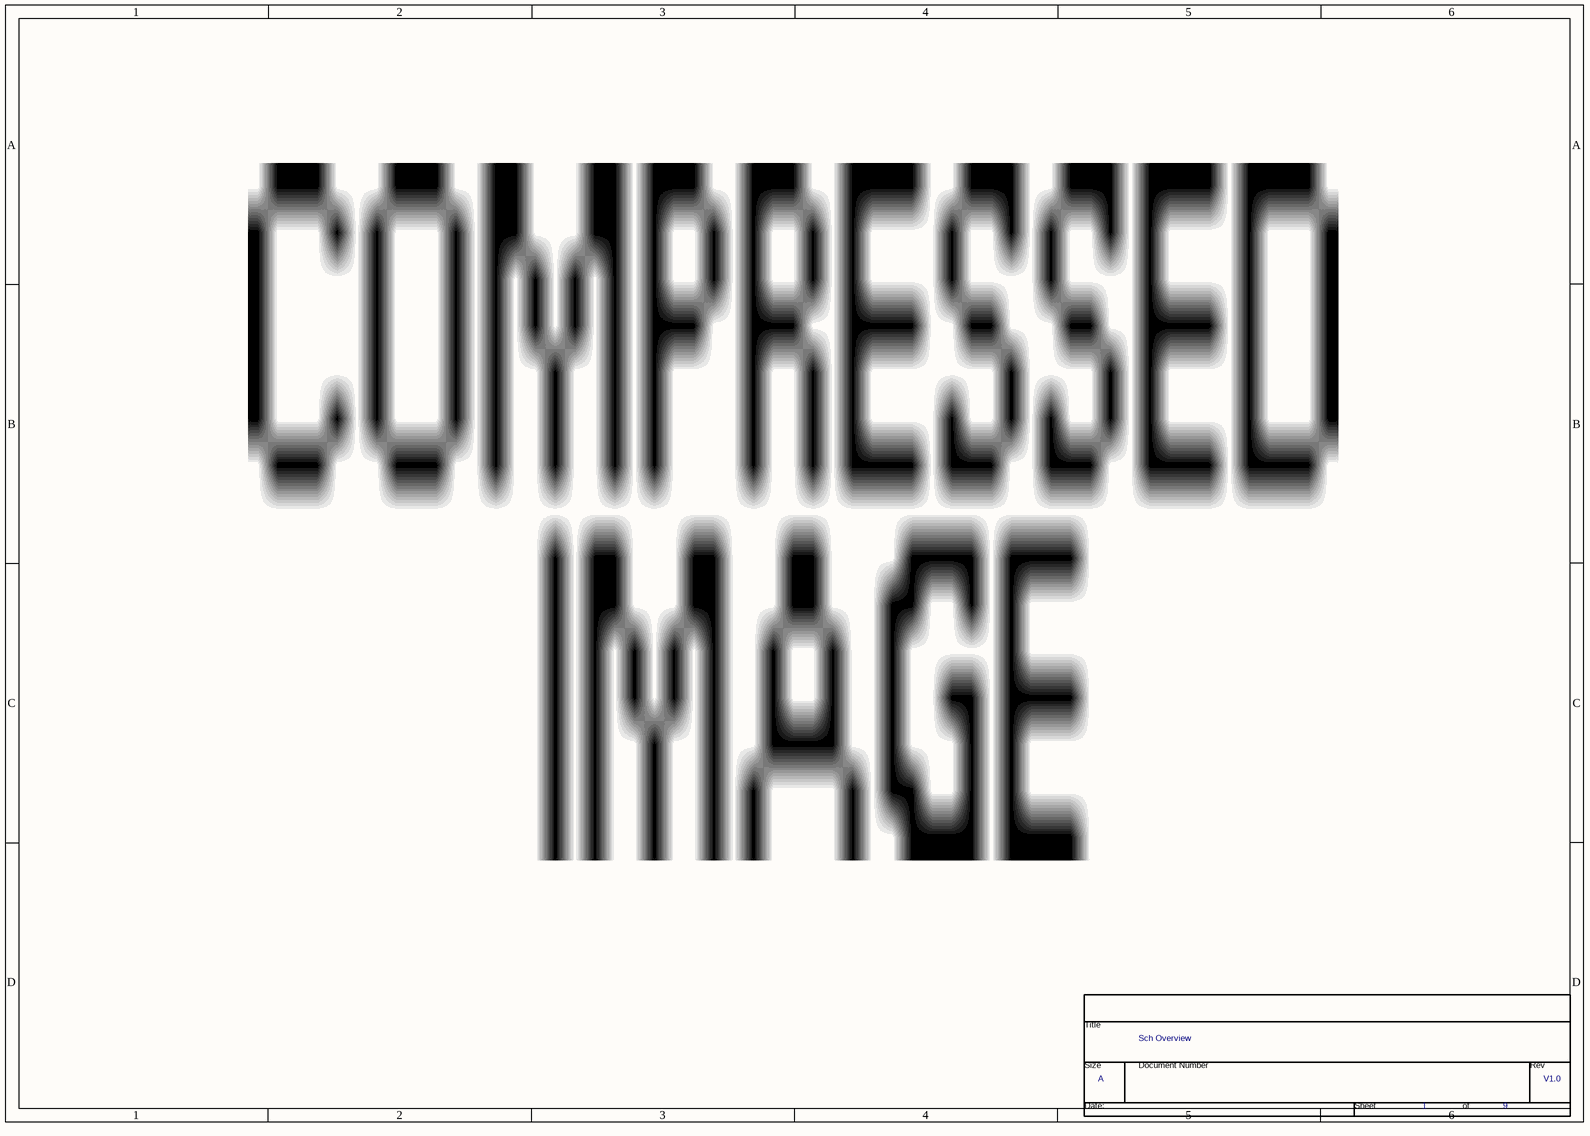
[diagram p0: MISC86294-2.SchDoc]
# Altium project MISC86294-22.PrjPcb (part 1 of 5)
9 sheets, 321 parts. Net scope: flat (ports and power ports of the same name join across sheets).
Board file: MISC86294.PcbDoc
Sheets:
  MISC86294-2.SchDoc
  MISC86294-4.SchDoc
  MISC86294-6.SchDoc
  MISC86294-8.SchDoc
  MISC86294-10.SchDoc
  MISC86294-12.SchDoc
  MISC86294-14.SchDoc
  MISC86294-16.SchDoc
  MISC86294-18.SchDoc

## Sheet MISC86294-2.SchDoc
size 297 x 209 mm

### Parts
(Parts that share a designator on the sheet are numbered #1, #2 ... from top to bottom, then left to right.)
*#1  RevCode: V1.0  Title: Sch Overview  Page Size: A  Page Number: 1  Page Count: 9  (hidden comment: TitleBlock0)  (graphical)

### Library data of the parts
*#1 = TitleBlock0: Document: Agr-Ctrl-3GS-01; Page Create Date: March  8, 1995

## Sheet MISC86294-4.SchDoc
size 297 x 209 mm
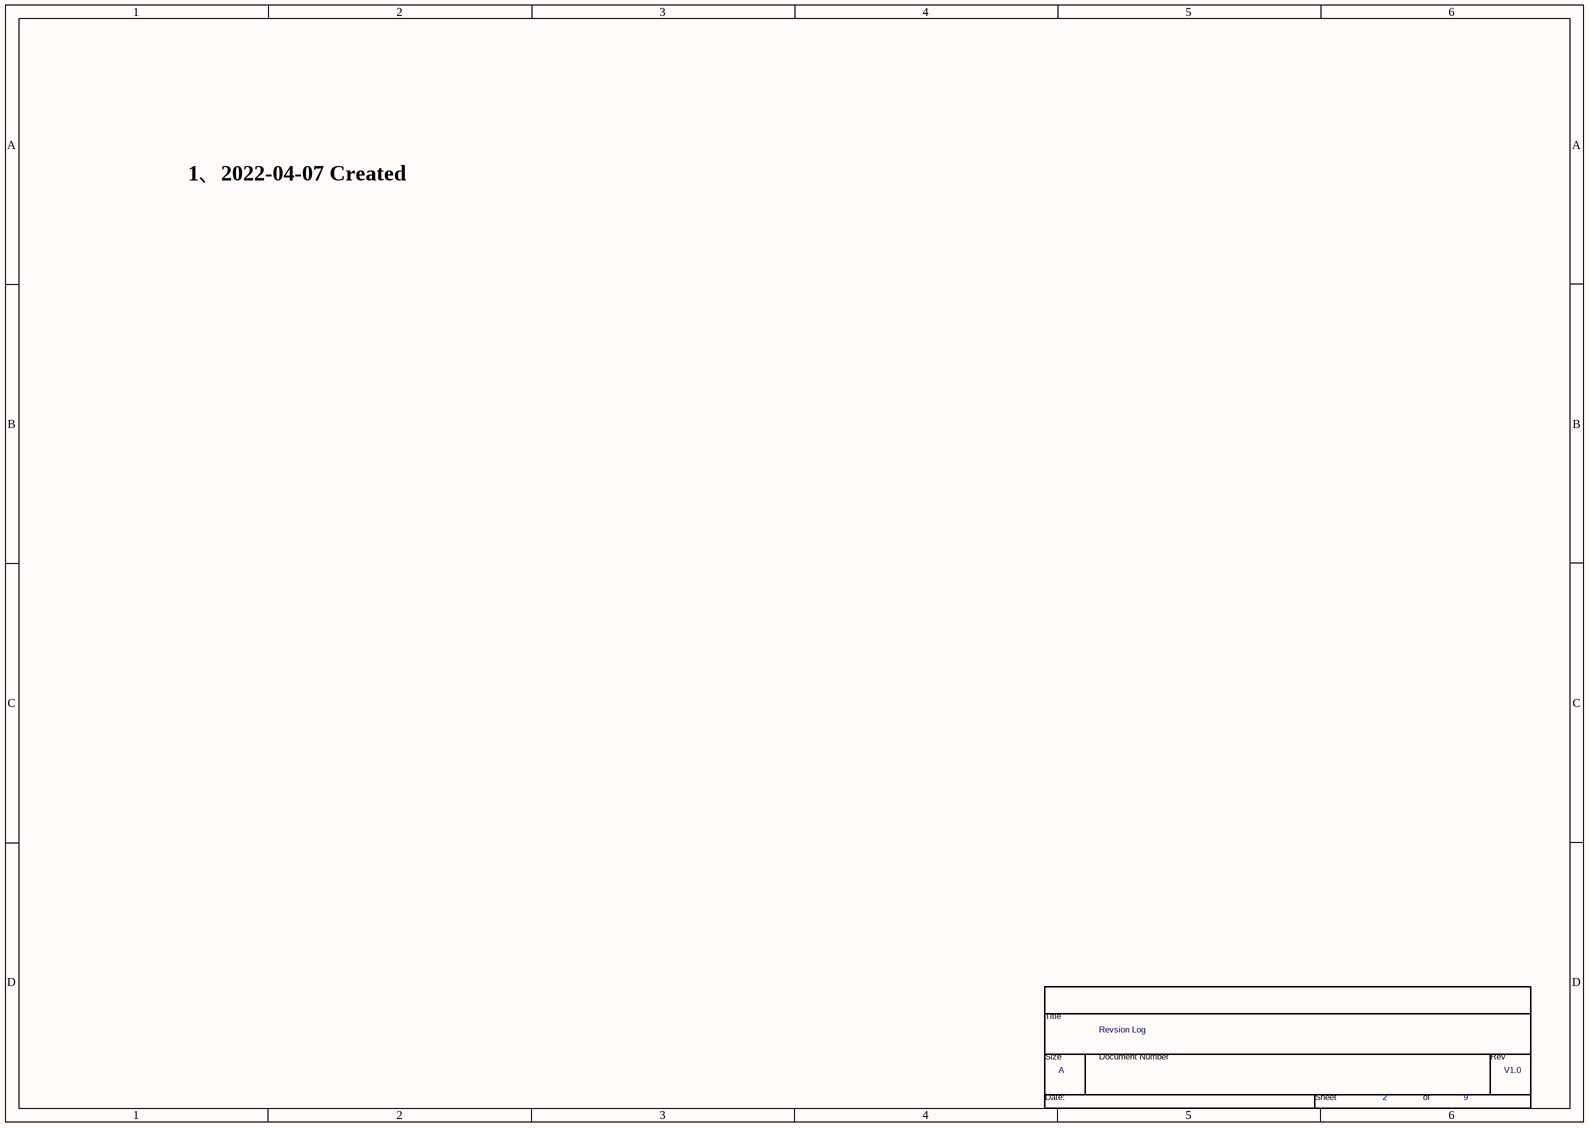
[diagram p1: MISC86294-4.SchDoc]

### Parts
(Parts that share a designator on the sheet are numbered #1, #2 ... from top to bottom, then left to right.)
*#2  RevCode: V1.0  Title: Revsion Log  Page Size: A  Page Number: 2  Page Count: 9  (hidden comment: TitleBlock0)  (graphical)

### Notes on the sheet
- 1、2022-04-07 Created

### Library data of the parts
*#2 = TitleBlock0: Document: Agr-Ctrl-3GS-02; Page Create Date: March  8, 1995

## Sheet MISC86294-6.SchDoc
size 297 x 209 mm
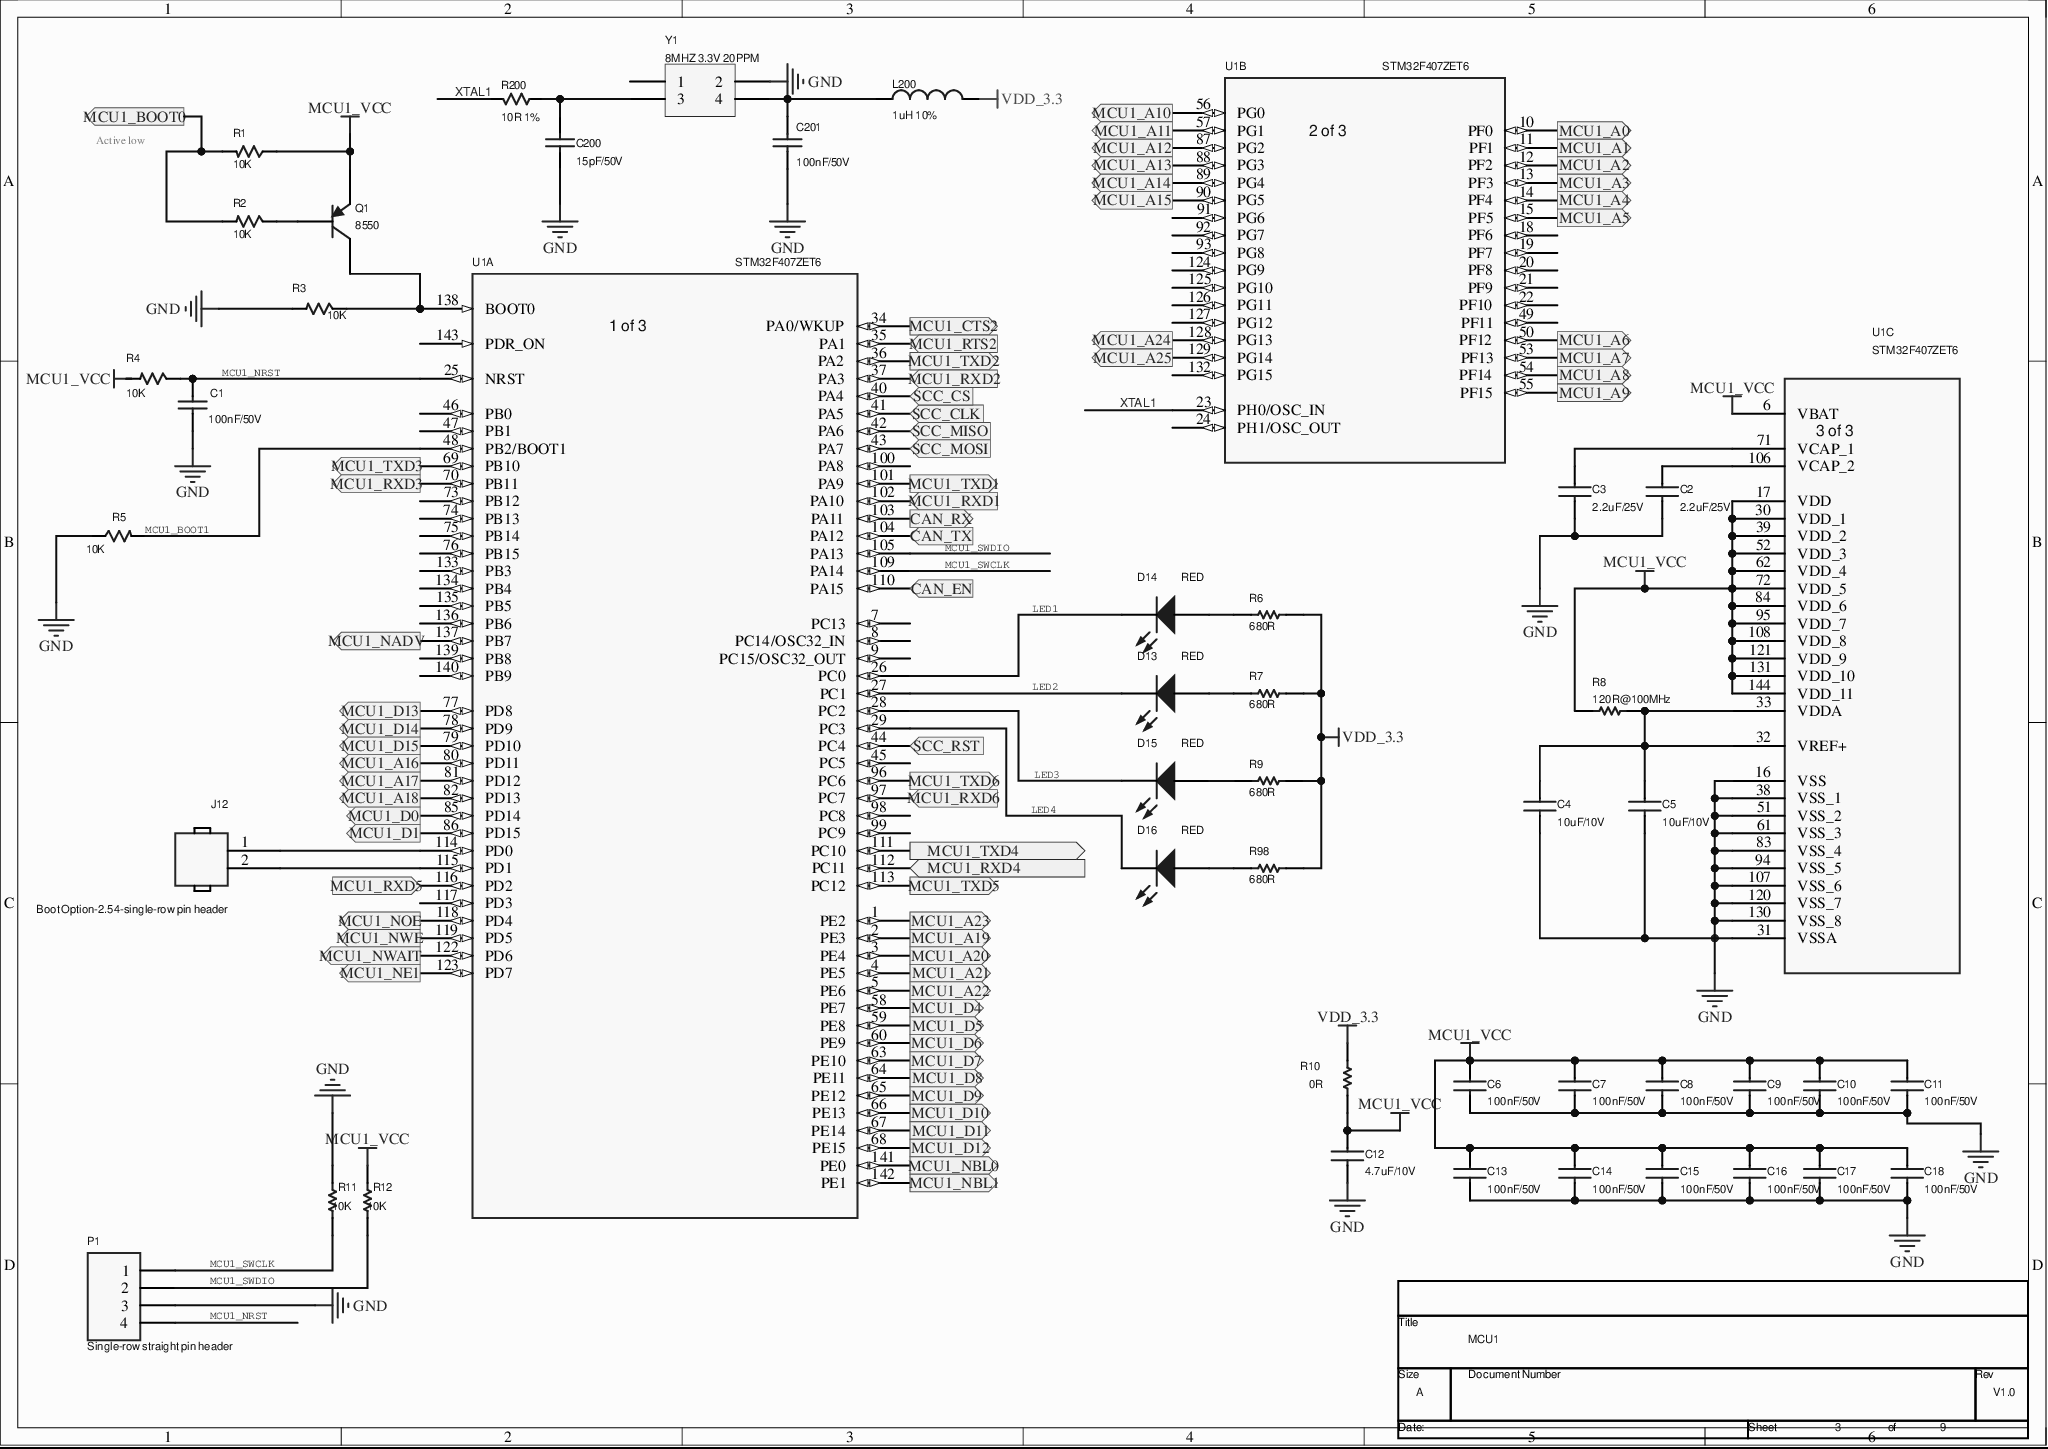
[diagram p2: MISC86294-6.SchDoc]

### Parts
(Parts that share a designator on the sheet are numbered #1, #2 ... from top to bottom, then left to right.)
*#3  RevCode: V1.0  Title: MCU1  Page Size: A  Page Number: 3  Page Count: 9  (hidden comment: TitleBlock0)  (graphical)
C1  100nF/50V  [0603]
C2  2.2uF/25V  [C0603]
C3  2.2uF/25V  [C0603]
C4  10uF/10V  [C0603]
C5  10uF/10V  [C0603]
C6  100nF/50V  [C0603]
C7  100nF/50V  [C0603]
C8  100nF/50V  [C0603]
C9  100nF/50V  [C0603]
C10  100nF/50V  [C0603]
C11  100nF/50V  [C0603]
C12  4.7uF/10V  [C0805]
C13  100nF/50V  [C0603]
C14  100nF/50V  [C0603]
C15  100nF/50V  [C0603]
C16  100nF/50V  [C0603]
C17  100nF/50V  [C0603]
C18  100nF/50V  [C0603]
C200  15pF/50V  [C0603]
C201  100nF/50V  [C0603]
D13  RED  [LED_0805]
D14  RED  [LED_0805]
D15  RED  [LED_0805]
D16  RED  [LED_0805]
J12  Boot Option-2.54-single-row pin header  [HDR_1X2_254]
L200  1uH 10%  [SMD_L6.0-W6.0]
P1  Single-row straight pin header  [HDR1X4]
Q1  8550  [SOT-23-SS8550]
R1  10K  [0603]
R2  10K  [0603]
R3  10K  [0603]
R4  10K  [0603]
R5  10K  [0603]
R6  User_Value: 680R  [0603]  (hidden comment: NA)
R7  User_Value: 680R  [0603]  (hidden comment: NA)
R8  120R@100MHz  [0603]
R9  User_Value: 680R  [0603]  (hidden comment: NA)
R10  0R  [0603]
R11  10K  [0603]
R12  10K  [0603]
R98  User_Value: 680R  [0603]  (hidden comment: NA)
R200  10R 1%  [R0805]
U1  STM32F407ZET6  [LQFP144-20x20mm]  (parts A,B,C of 3)
Y1  8MHZ 3.3V 20PPM  [XTAL 5.7X7.0-SM - duplicate]

### Ports
CAN_EN (in), CAN_RX (out), CAN_TX (in), MCU1_A0 (out), MCU1_A1 (out), MCU1_A2 (out), MCU1_A3 (out), MCU1_A4 (out), MCU1_A5 (out), MCU1_A6 (out), MCU1_A7 (out), MCU1_A8 (out), MCU1_A9 (out), MCU1_A10 (out), MCU1_A11 (out), MCU1_A12 (out), MCU1_A13 (out), MCU1_A14 (out), MCU1_A15 (out), MCU1_A16 (out), MCU1_A17 (out), MCU1_A18 (out), MCU1_A19 (out), MCU1_A20 (out), MCU1_A21 (out), MCU1_A22 (out), MCU1_A23 (out), MCU1_A24 (out), MCU1_A25 (out), MCU1_BOOT0 (out), MCU1_CTS2 (out), MCU1_D0 (out), MCU1_D1 (out), MCU1_D4 (out), MCU1_D5 (out), MCU1_D6 (out), MCU1_D7 (out), MCU1_D8 (out), MCU1_D9 (out), MCU1_D10 (out), MCU1_D11 (out), MCU1_D12 (out), MCU1_D13 (out), MCU1_D14 (out), MCU1_D15 (out), MCU1_NADV (out), MCU1_NBL0 (out), MCU1_NBL1 (out), MCU1_NE1 (out), MCU1_NOE (out), MCU1_NWAIT (out), MCU1_NWE (out), MCU1_RTS2 (in), MCU1_RXD1 (in), MCU1_RXD2 (in), MCU1_RXD3 (out), MCU1_RXD4 (in), MCU1_RXD5 (in), MCU1_RXD6 (in), MCU1_TXD1 (out), MCU1_TXD2 (out), MCU1_TXD3 (out), MCU1_TXD4 (out), MCU1_TXD5 (out), MCU1_TXD6 (out), SCC_CLK (in), SCC_CS (in), SCC_MISO (in), SCC_MOSI (in), SCC_RST (in)

### Nets
GND: C1.1 C2.2 C3.2 C4.2 C5.2 C6.2 C7.2 C8.2 C9.2 C10.2 C11.2 C12.2 C13.2 C14.2 C15.2 C16.2 C17.2 C18.2 C200.1 C201.2 P1.3 R3.1 R5.1 R11.2 U1.16(VSS) U1.31(VSSA) U1.38(VSS_1) U1.51(VSS_2) U1.61(VSS_3) U1.83(VSS_4) U1.94(VSS_5) U1.107(VSS_6) U1.120(VSS_7) U1.130(VSS_8) Y1.2
MCU1_VCC: C6.1 C7.1 C8.1 C9.1 C10.1 C11.1 C12.1 C13.1 C14.1 C15.1 C16.1 C17.1 C18.1 Q1.2(E) R1.2 R4.2 R8.1 R10.2 R12.2 U1.6(VBAT) U1.17(VDD) U1.30(VDD_1) U1.39(VDD_2) U1.52(VDD_3) U1.62(VDD_4) U1.72(VDD_5) U1.84(VDD_6) U1.95(VDD_7) U1.108(VDD_8) U1.121(VDD_9) U1.131(VDD_10) U1.144(VDD_11)
VDD_3.3: L200.2 R6.1 R7.1 R9.1 R10.1 R98.1
IMU_RXD1: U1.111(PC10) ; port MCU1_TXD4
IMU_TXD1: U1.112(PC11) ; port MCU1_RXD4
LED1: D14.2(K) U1.26(PC0)
LED2: D13.2(K) U1.27(PC1)
LED3: D15.2(K) U1.28(PC2)
LED4: D16.2(K) U1.29(PC3)
MCU1_BOOT1: R5.2 U1.48(PB2/BOOT1)
MCU1_NRST: C1.2 P1.4 R4.1 U1.25(NRST)
MCU1_SWCLK: P1.1 R11.1 U1.109(PA14)
MCU1_SWDIO: P1.2 R12.1 U1.105(PA13)
XTAL1: R200.1 U1.23(PH0/OSC_IN)
NetC2_1: C2.1 U1.106(VCAP_2)
NetC3_1: C3.1 U1.71(VCAP_1)
NetC4_1: C4.1 C5.1 R8.2 U1.32(VREF+) U1.33(VDDA)
NetC200_2: C200.2 R200.2 Y1.3
NetC201_1: C201.1 L200.1 Y1.4
NetD13_1: D13.1(A) R7.2
NetD14_1: D14.1(A) R6.2
NetD15_1: D15.1(A) R9.2
NetD16_1: D16.1(A) R98.2
NetJ6_39: U1.116(PD2) ; port MCU1_RXD5
NetJ6_40: U1.113(PC12) ; port MCU1_TXD5
NetJ12_1: J12.1 U1.114(PD0)
NetJ12_2: J12.2 U1.115(PD1)
NetJ13_1: U1.101(PA9) ; port MCU1_TXD1
NetJ13_2: U1.102(PA10) ; port MCU1_RXD1
NetJ14_1: U1.36(PA2) ; port MCU1_TXD2
NetJ14_2: U1.37(PA3) ; port MCU1_RXD2
NetJ16_1: U1.69(PB10) ; port MCU1_TXD3
NetJ16_2: U1.70(PB11) ; port MCU1_RXD3
NetJ22_1: U1.96(PC6) ; port MCU1_TXD6
NetJ22_2: U1.97(PC7) ; port MCU1_RXD6
NetP3_11: R1.1 R2.2 ; port MCU1_BOOT0
NetQ1_1: Q1.1(B) R2.1
NetQ1_3: Q1.3(C) R3.2 U1.138(BOOT0)
NetR23_1: U1.43(PA7) ; port SCC_MOSI
NetR24_1: U1.42(PA6) ; port SCC_MISO
NetU1_1: U1.1(PE2) ; port MCU1_A23
NetU1_2: U1.2(PE3) ; port MCU1_A19
NetU1_3: U1.3(PE4) ; port MCU1_A20
NetU1_4: U1.4(PE5) ; port MCU1_A21
NetU1_5: U1.5(PE6) ; port MCU1_A22
NetU1_10: U1.10(PF0) ; port MCU1_A0
NetU1_11: U1.11(PF1) ; port MCU1_A1
NetU1_12: U1.12(PF2) ; port MCU1_A2
NetU1_13: U1.13(PF3) ; port MCU1_A3
NetU1_14: U1.14(PF4) ; port MCU1_A4
NetU1_15: U1.15(PF5) ; port MCU1_A5
NetU1_34: U1.34(PA0/WKUP) ; port MCU1_CTS2
NetU1_35: U1.35(PA1) ; port MCU1_RTS2
NetU1_40: U1.40(PA4) ; port SCC_CS
NetU1_41: U1.41(PA5) ; port SCC_CLK
NetU1_44: U1.44(PC4) ; port SCC_RST
NetU1_50: U1.50(PF12) ; port MCU1_A6
NetU1_53: U1.53(PF13) ; port MCU1_A7
NetU1_54: U1.54(PF14) ; port MCU1_A8
NetU1_55: U1.55(PF15) ; port MCU1_A9
NetU1_56: U1.56(PG0) ; port MCU1_A10
NetU1_57: U1.57(PG1) ; port MCU1_A11
NetU1_58: U1.58(PE7) ; port MCU1_D4
NetU1_59: U1.59(PE8) ; port MCU1_D5
NetU1_60: U1.60(PE9) ; port MCU1_D6
NetU1_63: U1.63(PE10) ; port MCU1_D7
NetU1_64: U1.64(PE11) ; port MCU1_D8
NetU1_65: U1.65(PE12) ; port MCU1_D9
NetU1_66: U1.66(PE13) ; port MCU1_D10
NetU1_67: U1.67(PE14) ; port MCU1_D11
NetU1_68: U1.68(PE15) ; port MCU1_D12
NetU1_77: U1.77(PD8) ; port MCU1_D13
NetU1_78: U1.78(PD9) ; port MCU1_D14
NetU1_79: U1.79(PD10) ; port MCU1_D15
NetU1_80: U1.80(PD11) ; port MCU1_A16
NetU1_81: U1.81(PD12) ; port MCU1_A17
NetU1_82: U1.82(PD13) ; port MCU1_A18
NetU1_85: U1.85(PD14) ; port MCU1_D0
NetU1_86: U1.86(PD15) ; port MCU1_D1
NetU1_87: U1.87(PG2) ; port MCU1_A12
NetU1_88: U1.88(PG3) ; port MCU1_A13
NetU1_89: U1.89(PG4) ; port MCU1_A14
NetU1_90: U1.90(PG5) ; port MCU1_A15
NetU1_103: U1.103(PA11) ; port CAN_RX
NetU1_104: U1.104(PA12) ; port CAN_TX
NetU1_110: U1.110(PA15) ; port CAN_EN
NetU1_118: U1.118(PD4) ; port MCU1_NOE
NetU1_119: U1.119(PD5) ; port MCU1_NWE
NetU1_122: U1.122(PD6) ; port MCU1_NWAIT
NetU1_123: U1.123(PD7) ; port MCU1_NE1
NetU1_128: U1.128(PG13) ; port MCU1_A24
NetU1_129: U1.129(PG14) ; port MCU1_A25
NetU1_137: U1.137(PB7) ; port MCU1_NADV
NetU1_141: U1.141(PE0) ; port MCU1_NBL0
NetU1_142: U1.142(PE1) ; port MCU1_NBL1

Not connected (* = marked no-connect by the designer): U1 7(PC13) 8(PC14/OSC32_IN) 9(PC15/OSC32_OUT) 18(PF6) 19(PF7) 20(PF8) 21(PF9) 22(PF10) 24(PH1/OSC_OUT) 45(PC5) 46(PB0) 47(PB1) 49(PF11) 73(PB12) 74(PB13) 75(PB14) 76(PB15) 91(PG6) 92(PG7) 93(PG8) 98(PC8) 99(PC9) 100(PA8) 117(PD3) 124(PG9) 125(PG10) 126(PG11) 127(PG12) 132(PG15) 133(PB3) 134(PB4) 135(PB5) 136(PB6) 139(PB8) 140(PB9) 143(PDR_ON); Y1 1

### Notes on the sheet
- Active low

### Library data of the parts
*#3 = TitleBlock0: Document: Agr-Ctrl-3GS-03; Page Create Date: March  8, 1995
C1 = Cap_C14: Kind: General; SubKind: Capacitor; Origin: Altium; Published: 8-Jun-2000; Revision: July-2002: Re-released for DXP Platform.; User_Value: 100nF/50V; Spice Prefix: C; Type: Capacitor; Publisher: Altium Limited
C2-C18 = CAP NP_Dup1
C200 C201 = Cap: SMD capacitor; Published: 8-Jun-2000; Revision: July-2002: Re-released for DXP Platform.; Publisher: Altium Limited
  C200: Value: 15pF/50V
  C201: Value: 100nF/50V
D13-D16 = LED1_D4: Kind: General; SubKind: Diode; Origin: Altium; Published: 8-Jun-2000; LatestRevisionDate: 08-Jul-2005; LatestRevisionNote: Mech Layer 1 removed.; PackageReference: LED-1; Spice Prefix: D; Publisher: Altium Limited
J12 = HEADER 2
L200 = Inductor: SMD inductor; Code_IEC: 1005; Published: 8-Jun-2000; LatestRevisionDate: 17-Jul-2002; LatestRevisionNote: Re-released for DXP Platform.; PackageReference: 0402-A; Code_JEITA: 0402; Value: 1uH 10%; Publisher: Altium Limited
P1 = Header 4_P1: Origin: Altium; LatestRevisionDate: 17-Jul-2002; LatestRevisionNote: Re-released for DXP Platform.; Type: Connector; Publisher: Altium Limited
Q1 = PNP_Q1: Kind: Transistor; SubKind: BJT; Origin: Altium; Published: 8-Jun-2000; LatestRevisionDate: 29-May-2009; LatestRevisionNote: IPC-7351 Footprint Added.; PackageVersion: Aug-1999; PackageReference: SOT-23B; PackageDescription: 3-Pin SOT-23 Package 0.95 mm Pitch, 2.4 mm Lead Span; Created: 5/07/2006; Spice Prefix: Q; Type: BJT; Publisher: Altium Limited
R1 = Res_R2: Kind: General; SubKind: Resistor; Origin: Altium; Published: 8-Jun-2000; LatestRevisionDate: 04-Mar-2005; LatestRevisionNote: PCB Footprint replaced.; PackageReference: J1-0603; User_Value: 10K; Spice Prefix: R; Type: Resistor; Publisher: Altium Limited
R2 = Res_R3: Kind: General; SubKind: Resistor; Origin: Altium; Published: 8-Jun-2000; LatestRevisionDate: 04-Mar-2005; LatestRevisionNote: PCB Footprint replaced.; PackageReference: J1-0603; User_Value: 10K; Spice Prefix: R; Type: Resistor; Publisher: Altium Limited
R3 = Res_R4: Kind: General; SubKind: Resistor; Origin: Altium; Published: 8-Jun-2000; LatestRevisionDate: 04-Mar-2005; LatestRevisionNote: PCB Footprint replaced.; PackageReference: J1-0603; User_Value: 10K; Spice Prefix: R; Type: Resistor; Publisher: Altium Limited
R4 = Res_R5: Kind: General; SubKind: Resistor; Origin: Altium; Published: 8-Jun-2000; LatestRevisionDate: 04-Mar-2005; LatestRevisionNote: PCB Footprint replaced.; PackageReference: J1-0603; User_Value: 10K; Spice Prefix: R; Type: Resistor; Publisher: Altium Limited
R5 = Res_R1: Kind: General; SubKind: Resistor; Origin: Altium; Published: 8-Jun-2000; LatestRevisionDate: 04-Mar-2005; LatestRevisionNote: PCB Footprint replaced.; PackageReference: J1-0603; User_Value: 10K; Spice Prefix: R; Type: Resistor; Publisher: Altium Limited
R6 = Res1_R8: Origin: Altium; Published: 8-Jun-2000; LatestRevisionDate: 17-Jul-2002; LatestRevisionNote: Re-released for DXP Platform.; PackageReference: AXIAL-0.3; Publisher: Altium Limited
R7 = Res1_R10: Origin: Altium; Published: 8-Jun-2000; LatestRevisionDate: 17-Jul-2002; LatestRevisionNote: Re-released for DXP Platform.; PackageReference: AXIAL-0.3; Publisher: Altium Limited
R8 R10 = Res1_R21: Kind: General; SubKind: Resistor; Origin: Altium; Published: 8-Jun-2000; LatestRevisionDate: 17-Jul-2002; LatestRevisionNote: Re-released for DXP Platform.; PackageReference: AXIAL-0.3; Spice Prefix: R; Type: Resistor; Publisher: Altium Limited
  R8: User_Value: 120R@100MHz
  R10: User_Value: 0R
R9 R98 = Res1_R12: Origin: Altium; Published: 8-Jun-2000; LatestRevisionDate: 17-Jul-2002; LatestRevisionNote: Re-released for DXP Platform.; PackageReference: AXIAL-0.3; Publisher: Altium Limited
R11 = Res1_R6: Kind: General; SubKind: Resistor; Origin: Altium; Published: 8-Jun-2000; LatestRevisionDate: 17-Jul-2002; LatestRevisionNote: Re-released for DXP Platform.; PackageReference: AXIAL-0.3; User_Value: 10K; Spice Prefix: R; Type: Resistor; Publisher: Altium Limited
R12 = Res1_R7: Kind: General; SubKind: Resistor; Origin: Altium; Published: 8-Jun-2000; LatestRevisionDate: 17-Jul-2002; LatestRevisionNote: Re-released for DXP Platform.; PackageReference: AXIAL-0.3; User_Value: 10K; Spice Prefix: R; Type: Resistor; Publisher: Altium Limited
R200 = Res: SMD resistor; Published: 8-Jun-2000; LatestRevisionDate: 04-Mar-2005; LatestRevisionNote: PCB Footprint replaced.; PackageReference: J1-0603; Value: 10R 1%; Publisher: Altium Limited
U1 = STM32F407ZET6: Mfr_Name: STMicroelectronics; Manufacturer_Part_Number: STM32F407ZET6; Copyright: Copyright (C) 2022 Ultra Librarian. All rights reserved.
Y1 = Header 2X2: Header, 2-Pin, Dual row; LatestRevisionDate: 17-Jul-2002; LatestRevisionNote: Re-released for DXP Platform.; Publisher: Altium Limited